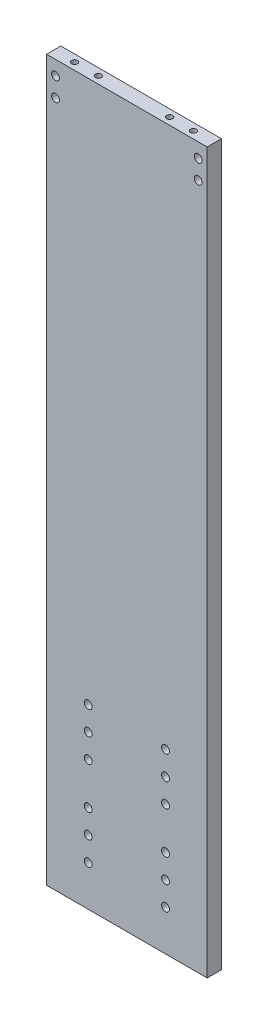
from build123d import *

# Parameters (mm, degrees)
SKETCH_1_W                  = 135
SKETCH_1_H                  = 605
EXTRUDE_1_DEPTH             = 6
HOLE_WIZARD_M6_1_D          = 5
HOLE_WIZARD_M6_1_DEPTH      = 17
HOLE_WIZARD_M6_1_TIP        = 1.502151548
HOLE_WIZARD_2_D             = 6.6
HOLE_WIZARD_2_CBORE_D       = 11
HOLE_WIZARD_2_CBORE_DEPTH   = 6.8
HOLE_WIZARD_2_2_D           = 6.6
HOLE_WIZARD_2_2_CBORE_D     = 11
HOLE_WIZARD_2_2_CBORE_DEPTH = 6.8


with BuildPart() as part:
    # 草图1 → 凸台-拉伸1 (new, symmetric)
    with BuildSketch(Plane.XY):
        Rectangle(SKETCH_1_W, SKETCH_1_H)
    extrude(amount=EXTRUDE_1_DEPTH, both=True)

    # M6 螺纹孔1
    with Locations(Plane(origin=(0, 302.5, 0), x_dir=(1, 0, 0), z_dir=(0, 1, 0))):
        with Locations((50, 0), (-30, 0), (30, 0), (-405, -6), (-50, 0)):
            Hole(HOLE_WIZARD_M6_1_D / 2, depth=HOLE_WIZARD_M6_1_DEPTH)
            with Locations((0, 0, -(HOLE_WIZARD_M6_1_DEPTH + HOLE_WIZARD_M6_1_TIP / 2))):  # 118° drill point
                Cone(0, HOLE_WIZARD_M6_1_D / 2, HOLE_WIZARD_M6_1_TIP, mode=Mode.SUBTRACT)

    # Hole Wizard 2 (through all)
    with Locations(Plane(origin=(0, 0, -6), x_dir=(-1, 0, 0), z_dir=(0, 0, -1))):
        with Locations((-60, 290.5), (60, 290.5), (-60, 274.5), (60, 274.5)):
            CounterBoreHole(HOLE_WIZARD_2_D / 2, HOLE_WIZARD_2_CBORE_D / 2, HOLE_WIZARD_2_CBORE_DEPTH)

    # Hole Wizard 2 2 (through all)
    with Locations(Plane(origin=(0, 0, -6), x_dir=(-1, 0, 0), z_dir=(0, 0, -1))):
        with Locations((-32.5, -153.5), (-32.5, -228.5), (32.5, -228.5), (32.5, -153.5), (32.5, -173.5), (32.5, -248.5), (-32.5, -248.5), (-32.5, -173.5), (32.5, -268.5), (32.5, -193.5), (-32.5, -193.5), (-32.5, -268.5)):
            CounterBoreHole(HOLE_WIZARD_2_2_D / 2, HOLE_WIZARD_2_2_CBORE_D / 2, HOLE_WIZARD_2_2_CBORE_DEPTH)


solid = part.part
